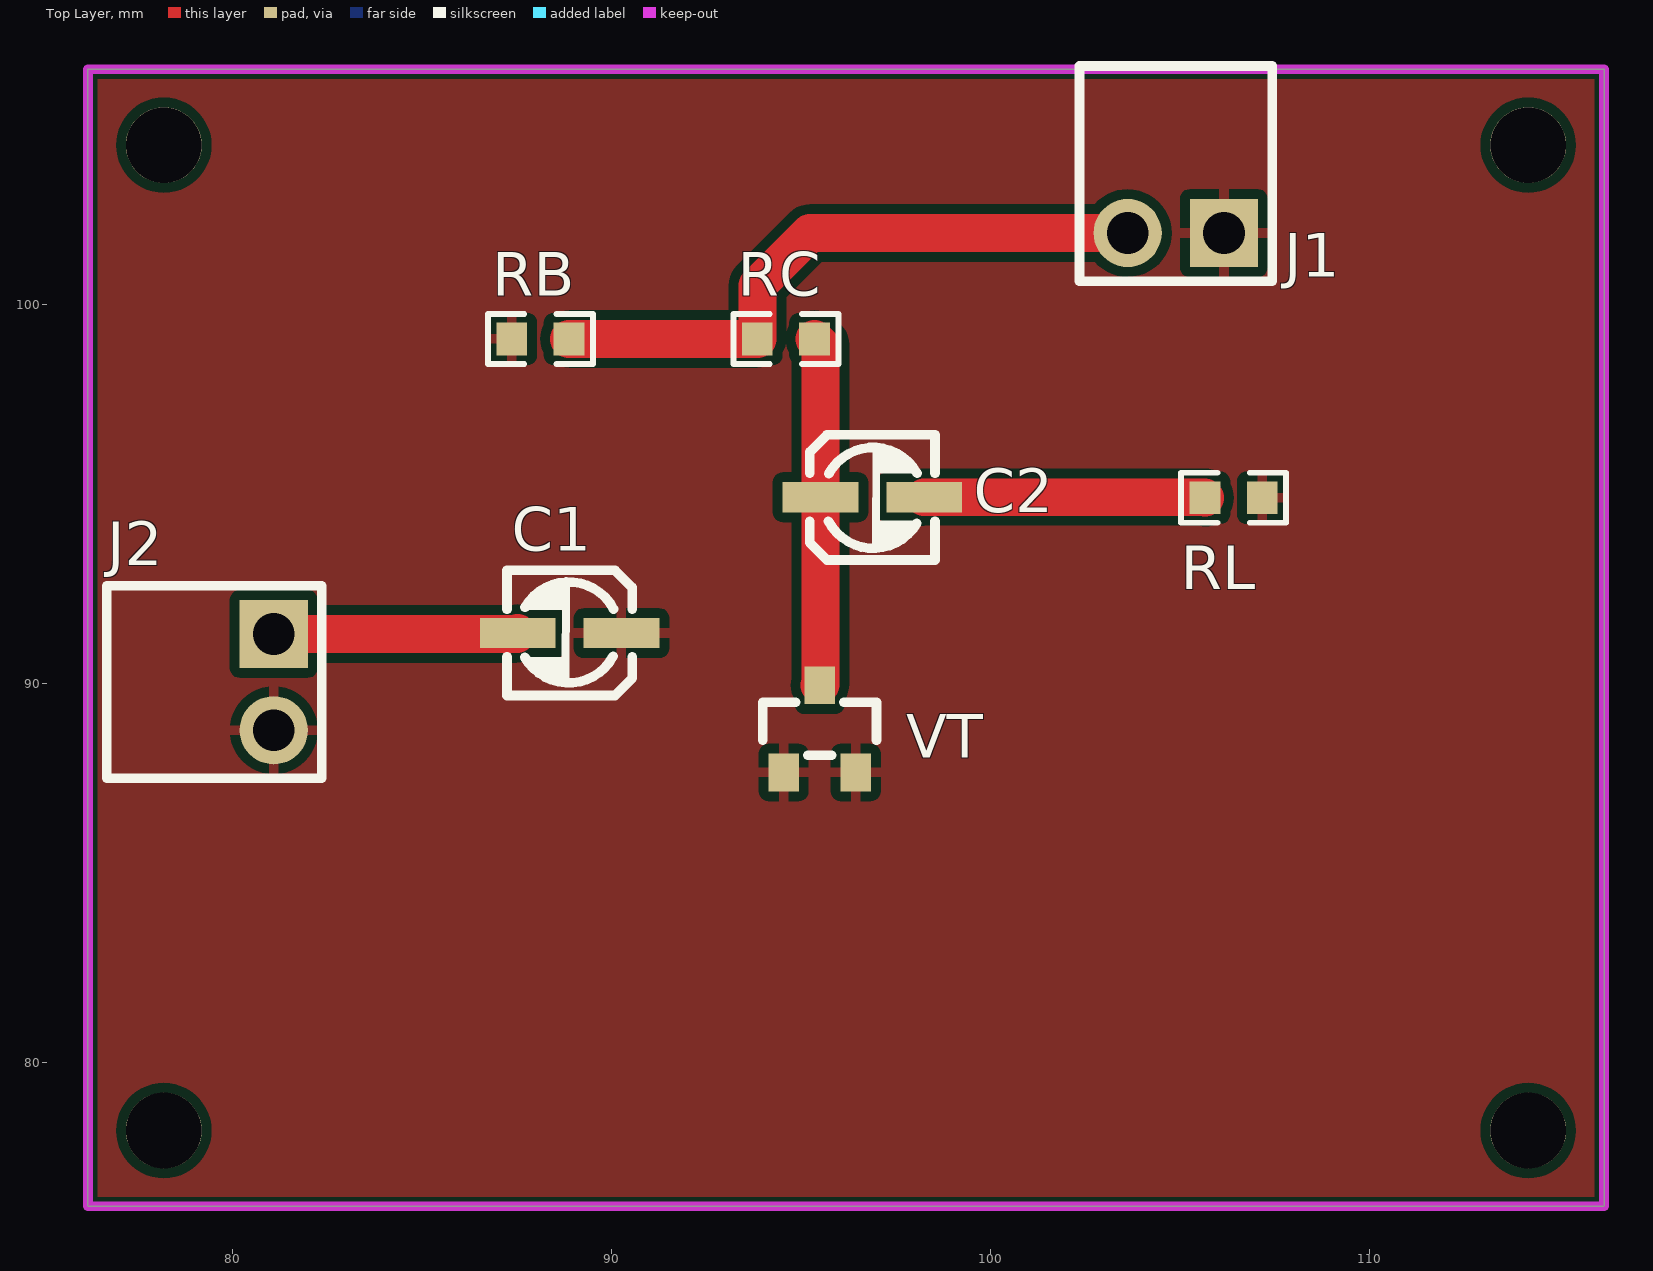
[diagram p0: Top Layer view]
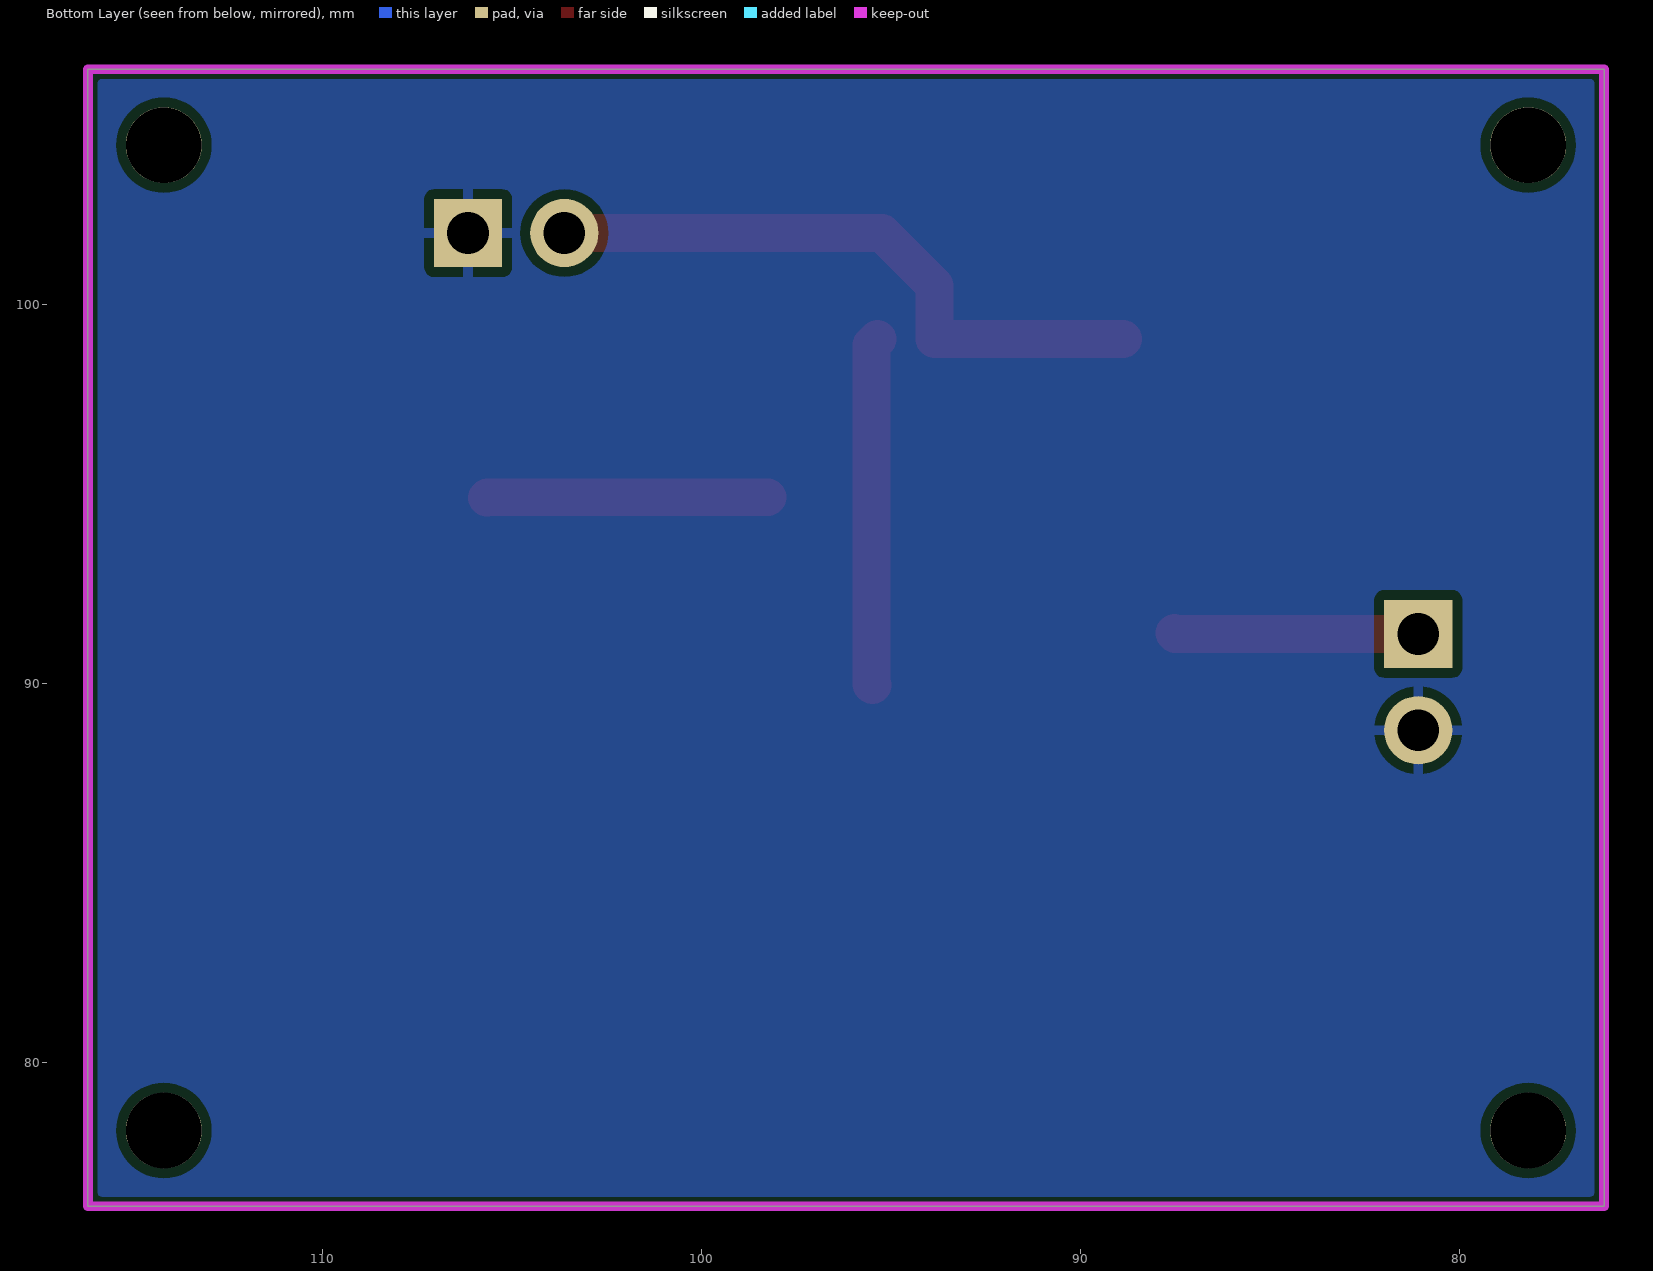
[diagram p1: Bottom Layer view, seen from below]
# Altium PCB MISC51134.pcbdoc
Units mm, origin at the board's own origin, x right, y up, seen from the top; angles counter-clockwise.
Board outline 40 x 30 mm, 2 copper layers (Top Layer, Bottom Layer), stack 1.58 mm thick; 8 components, 5 nets, 21 pads, 0 vias.

## Layer stack, top to bottom
Top Solder Mask Layer: solder mask 0.01, Dk 3.3
Top Layer: signal copper 0.035
Dielectric1: surface 1.51, FR4, Dk 4.5
Bottom Layer: signal copper 0.035
Bottom Solder Mask Layer: solder mask 0.01, Dk 3.3

## Board outline
76.2,106.2 76.2,76.2 116.2,76.2 116.2,106.2

## Design rules (kind name [scope] priority, off if disabled: settings)
BoardOutlineClearance copperThickness2oz_1 [All] p2 off: genericclearance=0.203 ignorepadtopadclearanceinfootprint=FALSE except(0: Arc-SplitContinuation Track-SplitContinuation SMDPad-SplitContinuation THPad-SplitContinuation Via-SplitContinuation Fill-SplitContinuation Region-SplitContinuation Poly-SplitContinuation Text-SplitContinuation Hole-SplitContinuation; 0.152: Arc-CutoutEdge SMDPad-CutoutEdge THPad-CutoutEdge Via-CutoutEdge Fill-CutoutEdge Region-CutoutEdge Text-CutoutEdge; 0.176: Hole-OutlineEdge Hole-CutoutEdge; 0.254: Poly-OutlineEdge Poly-CutoutEdge; 0.3: Arc-OutlineEdge Track-OutlineEdge SMDPad-OutlineEdge THPad-OutlineEdge Via-OutlineEdge Fill-OutlineEdge Region-OutlineEdge Text-OutlineEdge Track-CutoutEdge)
BoardOutlineClearance copperThickness1oz_1 [All] p4: genericclearance=0.102 ignorepadtopadclearanceinfootprint=FALSE except(0: Arc-SplitContinuation Track-SplitContinuation SMDPad-SplitContinuation THPad-SplitContinuation Via-SplitContinuation Fill-SplitContinuation Region-SplitContinuation Poly-SplitContinuation Text-SplitContinuation Hole-SplitContinuation; 0.152: SMDPad-CutoutEdge THPad-CutoutEdge Via-CutoutEdge Fill-CutoutEdge Region-CutoutEdge Text-CutoutEdge; 0.176: Hole-OutlineEdge Hole-CutoutEdge; 0.254: Poly-OutlineEdge Poly-CutoutEdge; 0.3: Arc-OutlineEdge Track-OutlineEdge SMDPad-OutlineEdge THPad-OutlineEdge Via-OutlineEdge Fill-OutlineEdge Region-OutlineEdge Text-OutlineEdge Arc-CutoutEdge Track-CutoutEdge)
Clearance copperThickness2oz [All] p1 off: gap=0.203 ignorepadtopadclearanceinfootprint=FALSE except(0.152: SMDPad-Track SMDPad-SMDPad THPad-Track SMDPad-THPad THPad-THPad Track-Via SMDPad-Via THPad-Via Via-Via Fill-Track Region-Track Fill-SMDPad Region-SMDPad Fill-THPad Region-THPad Fill-Via Region-Via Fill-Fill Fill-Region Region-Region Arc-Track Arc-SMDPad Arc-THPad Arc-Via Fill-Arc Region-Arc Arc-Arc Text-Track SMDPad-Text Text-THPad Text-Via Fill-Text Region-Text Arc-Text Text-Text; 0.176: Hole-Track Hole-SMDPad Hole-THPad Hole-Via Fill-Hole Region-Hole Hole-Arc Hole-Text; 0.254: Poly-Track Poly-SMDPad Poly-THPad Poly-Via Poly-Fill Poly-Region Poly-Poly Poly-Arc Poly-Text Poly-Hole)
Clearance copperThickness1oz [All] p3: gap=0.102 ignorepadtopadclearanceinfootprint=FALSE except(0.152: SMDPad-Track SMDPad-SMDPad THPad-Track SMDPad-THPad THPad-THPad Track-Via SMDPad-Via THPad-Via Via-Via Fill-Track Region-Track Fill-SMDPad Region-SMDPad Fill-THPad Region-THPad Fill-Via Region-Via Fill-Fill Fill-Region Region-Region Arc-Track Arc-SMDPad Arc-THPad Arc-Via Fill-Arc Region-Arc Arc-Arc Text-Track SMDPad-Text Text-THPad Text-Via Fill-Text Region-Text Arc-Text Text-Text; 0.176: Hole-Track Hole-SMDPad Hole-THPad Hole-Via Fill-Hole Region-Hole Hole-Arc Hole-Text; 0.254: Poly-Track Poly-SMDPad Poly-THPad Poly-Via Poly-Fill Poly-Region Poly-Poly Poly-Arc Poly-Text Poly-Hole)
Creepage creepage [All] p1: checkdistance=0 ignoreinternallayers=TRUE applytopolygonpour=TRUE
DiffPairsRouting differentialPair [All] p1: maxlimit=0.152 minlimit=0.152 mostfreqgap=0.152 toplayer_minwidth=0.127 toplayer_prefwidth=0.254 toplayer_maxwidth=2.54 toplayer_mingap=0.152 toplayer_prefgap=0.152 toplayer_maxgap=0.152 bottomlayer_minwidth=0.127 bottomlayer_prefwidth=0.254 bottomlayer_maxwidth=2.54 bottomlayer_mingap=0.152 bottomlayer_prefgap=0.152 bottomlayer_maxgap=0.152 maxuncoupledlength=0.254
HoleToHoleClearance otherClearance [All] p1: gap=0.3 allowstackedmicrovias=TRUE
Length netLength [All] p1: minlimit=0 maxlimit=0
MatchedLengths netLengthTolerance [All] p1: tolerance=25.4
PasteMaskExpansion pasteMaskExpansion [All] p1: expansion=0
PlaneConnect innerPlane [All] p1: planeconnectstyle=Relief reliefexpansion=0.508 reliefentries=4 reliefconductorwidth=0.254 reliefairgap=0.254
PolygonConnect copperRegion [(InNet('GND'))] p1: connectstyle=Relief reliefconductorwidth=0.254 reliefentries=4 polygonreliefangle="90 Angle" airgapwidth=0.254 via.connectstyle=Relief via.reliefconductorwidth=0.254 via.reliefentries=4 via.polygonreliefangle="90 Angle" via.airgapwidth=0.254
RoutingVias viaSize [All] p1: holewidth=0.305 width=0.61 viastyle="Through Hole" minholewidth=0.3 minwidth=0.5 maxholewidth=6.3 maxwidth=10
SolderMaskExpansion solderMaskExpansion [IsVia] p1: expansion=-25.4 istentingtop=TRUE
SolderMaskExpansion solderMaskExpansion [All] p2: expansion=0.051 istentingtop=FALSE
Width copperThickness2oz_2 [All] p1 off: maxlimit=2.54 minlimit=0.203 preferedwidth=0.254
Width copperThickness1oz_2 [All] p2: maxlimit=2.54 minlimit=0.127 preferedwidth=0.254

## Components (designator, comment, footprint, x,y, rotation, side; value= is the part's Value field where it differs from the comment)
C1 "100pF" C_Ele_SMD_3x5.4mm 88.9,91.341 r0 top
C2 "100pF" C_Ele_SMD_3x5.4mm 96.901,94.897 r180 top
J1 "" HDR-TH_2P-P2.54-V-M-1 104.902,101.882 r180 top
J2 "" HDR-TH_2P-P2.54-V-M-1 81.101,90.032 r270 top
RB "5.1K" R0603 88.138,99.088 r0 top
RC "1K" R0603 94.615,99.088 r180 top
RL "1K" R0603 106.426,94.897 r180 top
VT "" S8050_SOT-23 95.504,88.801 r270 top

## Footprints (in the part's own frame and the unit in brackets; to place one, negate y for a bottom-side part, rotate by r counter-clockwise, add the part's x,y. Pads: shape width x height; smd on the part's side, far side on the other; paste and mask are expansions set on the pad)
C_Ele_SMD_3x5.4mm [mil]
  rect 78.7x31.5 smd paste+0 mask+2: 1(54.1,-0.55) 2(-53.7,-0.55)
  silkscreen extent -65,-65 65,65
HDR-TH_2P-P2.54-V-M-1 [mm]
  rect 1.8x1.8 hole 1.1: 1(-1.27,0)
  round 1.8 hole 1.1: 2(1.27,0)
  silkscreen extent -2.54,-4.41 2.54,1.27
R0603 [mm]
  rect 0.806x0.864 smd paste-100 mask+0.051: 1(-0.753,0) 2(0.753,0)
  silkscreen extent -1.39,-0.66 1.39,0.66
S8050_SOT-23 [mm]
  rect 1x0.8 smd paste+0 mask+0.051: 1(1.15,-0.95) 2(1.15,0.95) 3(-1.15,0)
  silkscreen extent -0.7,-1.5 0.7,1.5

## Free pads (board coordinates)
  round 2 hole 2: 1(78.2,78.2) 1(78.2,104.2) 1(114.2,78.2) 1(114.2,104.2)

## Nets (pads, with @x,y where several pads share a name; then routed paths per layer and width w, separated by ;. In a path a pad name is that pad's centre, name@x,y a point inside that pad or via, vN(x,y) a via of type N, cw(c..) or ccw(c..) an arc to the next point about the centre after c; other vN are vias at no path point)
$1N24: C1.2 J2.1 | length 6.4
  Top Layer w1: J2.1 87.511,91.302 C1.2
$1N29: C2.1 RC.1 VT.3 | length 9.2
  Top Layer w1: RC.1 95.527,98.93 C2.1 95.527,89.974 VT.3
$1N31: C2.2 RL.2 | length 7.4
  Top Layer w1: C2.2 105.659,94.911 RL.2
EC: J1.2 RB.2 RC.2 | length 16.7
  Top Layer w1: RB.2 RC.2 93.862,100.494 95.25,101.882 J1.2
GND: C1.1 J1.1 J2.2 RB.1 RL.1 VT.1 VT.2

## Polygon pours and split planes (outlines as drawn)
GND on Top Layer (solid, remove dead copper, pour order 0): 76.2,106.2 76.2,76.2 116.2,76.2 116.2,106.2
GND on Bottom Layer (solid, remove dead copper, pour order 2): 76.2,106.2 76.2,76.2 116.2,76.2 116.2,106.2

## Keep-outs
Board Outline Layer:
  the board outline again, w0.254